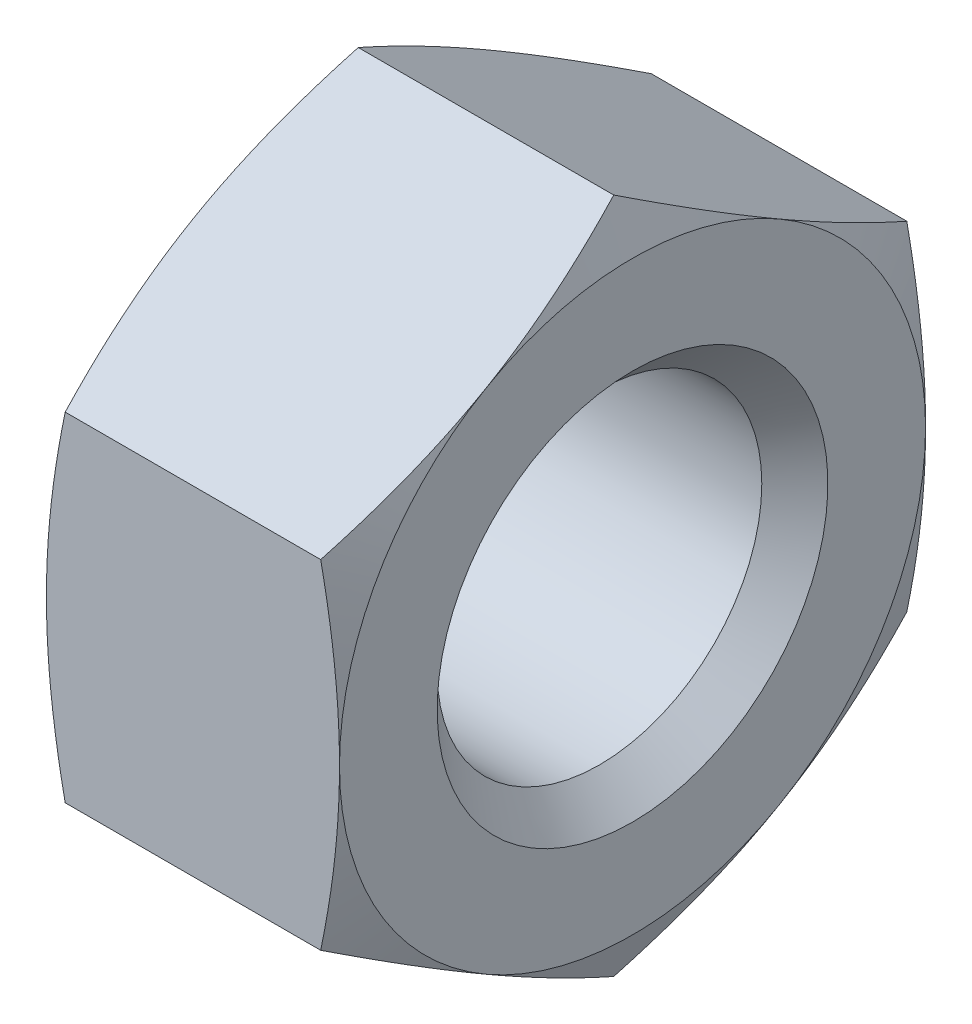
from build123d import *

# Parameters (mm, degrees)
CUT_EXTRUDE_1_DEPTH      = 3
CUT_EXTRUDE_1_DEPTH_BACK = 3
SKETCH_2_R               = 45
SCALE_1_SCALE            = 0.5


with BuildPart() as part:
    # 草图1 → 旋转1 (revolve)
    with BuildSketch(Plane.XY, mode=Mode.PRIVATE) as revolve_1_sk:
        Polygon((-3, 6), (-3, 4), (-2.3235, 3.3235), (2.3235, 3.3235), (3, 4), (3, 6), (0, 13.242640687), align=None)
    revolve(revolve_1_sk.sketch.rotate(Axis((3, 0, 0), (-1, 0, 0)), 180), axis=Axis((3, 0, 0), (-1, 0, 0)))

    # 草图2 → 切除-拉伸1 (cut, two sides: drawn at the far end of the back side and taken through both)
    with BuildSketch(Plane(origin=(0, 0, 0), x_dir=(0, 0, -1), z_dir=(1, 0, 0)).offset(-CUT_EXTRUDE_1_DEPTH_BACK)):
        Circle(SKETCH_2_R)
        Polygon((-6, -3.464101615), (0, -6.92820323), (6, -3.464101615), (6, 3.464101615), (0, 6.92820323), (-6, 3.464101615), align=None, mode=Mode.SUBTRACT)
    extrude(amount=CUT_EXTRUDE_1_DEPTH + CUT_EXTRUDE_1_DEPTH_BACK, mode=Mode.SUBTRACT)


with BuildPart() as part_1:
    # 缩放比例1: scaled about (0, 1e-09, 0)
    add(part.part.scale(SCALE_1_SCALE).moved(Location((0, 1e-09, 0))))


solid = part_1.part
